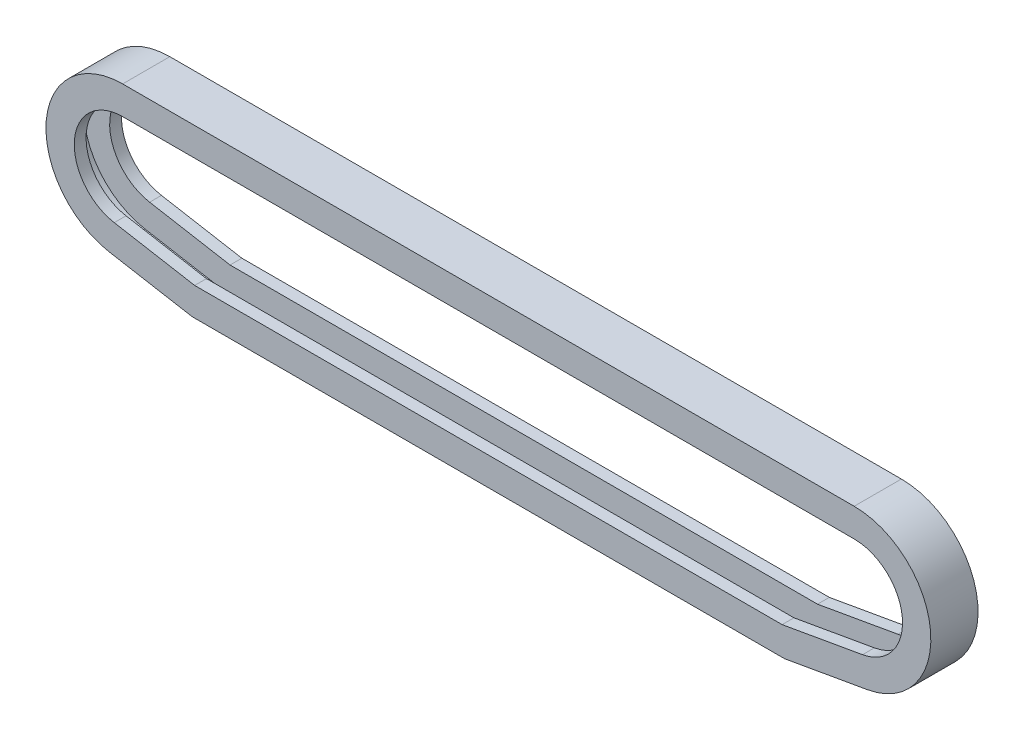
SolidWorks part; units mm, degrees
ref_plane "Front Plane" through (0, 0, 0) normal (0, 0, 1) x (1, 0, 0)
ref_plane "Top Plane" through (0, 0, 0) normal (0, 1, 0) x (1, 0, 0)
ref_plane "Right Plane" through (0, 0, 0) normal (1, 0, 0) x (0, 0, -1)
sketch "Sketch2" plane through (0, 0, 0) normal (0, 0, 1) x (1, 0, 0)
  line L0 (155, 0) -> (-155, 0) construction
  line L1 (0, 0) -> (0, -32.1986) construction
  line L2 (-125, -32.1986) -> (-159.6017, -26.0974) construction
  line L3 (125, -32.1986) -> (159.6017, -26.0974) construction
  line L4 (-155, 26.5) -> (155, 26.5) construction
  line L5 (-125, -32.1986) -> (125, -32.1986) construction
  line L6 (-155, 0) -> (-159.6017, -26.0974) construction
  line L7 (-155, 32.5) -> (155, 32.5)
  line L8 (125.5249, -38.1986) -> (160.6436, -32.0063)
  line L9 (-125.5249, -38.1986) -> (125.5249, -38.1986)
  line L10 (-125.5249, -38.1986) -> (-160.6436, -32.0063)
  line L11 (-155, 20.5) -> (155, 20.5)
  line L12 (124.4751, -26.1986) -> (158.5598, -20.1886)
  line L13 (-124.4751, -26.1986) -> (124.4751, -26.1986)
  line L14 (-124.4751, -26.1986) -> (-158.5598, -20.1886)
  arc A0 (-155, 26.5) -> (-159.6017, -26.0974) centre (-155, 0) ccw construction
  arc A1 (155, 26.5) -> (159.6017, -26.0974) centre (155, 0) cw construction
  arc A2 (155, 32.5) -> (160.6436, -32.0063) centre (155, 0) cw
  arc A3 (-155, 32.5) -> (-160.6436, -32.0063) centre (-155, 0) ccw
  arc A4 (155, 20.5) -> (158.5598, -20.1886) centre (155, 0) cw
  arc A5 (-155, 20.5) -> (-158.5598, -20.1886) centre (-155, 0) ccw
  point P6 (0, 0)
  dimension "D1" = 53
  dimension "D7" = 32.5
  dimension "D8" = 20.5
  dimension "D2" = 310
  dimension "D3" = 30
  dimension "D4" = 100
  dimension "D5" = 6
  dimension "D6" = 6
extrude "Boss-Extrude1" add sketch "Sketch2" along normal mid plane 20
sketch "Sketch8" plane through (0, 0, 0) normal (0, 0, 1) x (1, 0, 0)
  line L18 (125.4374, -37.1986) -> (160.4699, -31.0214)
  line L19 (-125.4374, -37.1986) -> (125.4374, -37.1986)
  line L20 (-160.4699, -31.0214) -> (-125.4374, -37.1986)
  line L21 (155, 31.5) -> (-155, 31.5)
  line L22 (125.4374, -37.1986) -> (160.4699, -31.0214)
  line L23 (-125.4374, -37.1986) -> (125.4374, -37.1986)
  line L24 (-160.4699, -31.0214) -> (-125.4374, -37.1986)
  line L25 (155, 31.5) -> (-155, 31.5)
  arc A12 (160.4699, -31.0214) -> (155, 31.5) centre (155, 0) ccw
  arc A13 (-155, 31.5) -> (-160.4699, -31.0214) centre (-155, 0) ccw
  arc A14 (160.4699, -31.0214) -> (155, 31.5) centre (155, 0) ccw
  arc A15 (-155, 31.5) -> (-160.4699, -31.0214) centre (-155, 0) ccw
  dimension "D1" = 1
extrude "Cut-Extrude1" cut sketch "Sketch8" against normal mid plane 10
